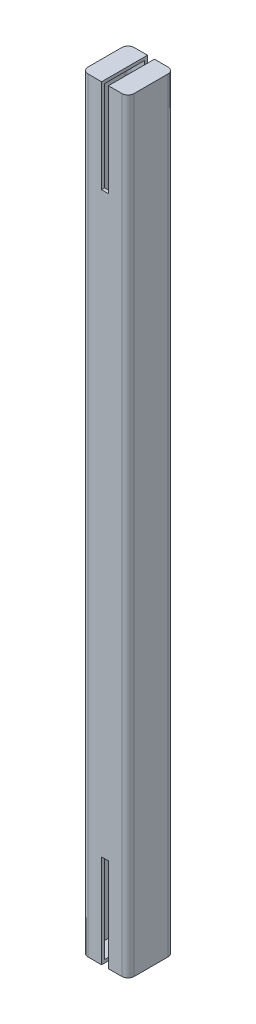
SolidWorks part; units mm, degrees
material "Q235B"
ref_plane "Front Plane" through (0, 0, 0) normal (0, 0, 1) x (1, 0, 0)
ref_plane "Top Plane" through (0, 0, 0) normal (0, 1, 0) x (1, 0, 0)
ref_plane "Right Plane" through (0, 0, 0) normal (1, 0, 0) x (0, 0, -1)
other "Configuration Table"
sketch "Sketch1" plane through (0, 0, 0) normal (0, 1, 0) x (1, 0, 0)
  line L0 (-22, 26) -> (22, 26)
  line L1 (-22, -30) -> (22, -30)
  line L2 (-30, -22) -> (-30, 22)
  line L3 (-22, 30) -> (22, 30)
  line L4 (30, -22) -> (30, 22)
  line L5 (-30, -30) -> (30, 30) construction
  line L6 (-30, 30) -> (30, -30) construction
  line L7 (26, -22) -> (26, 22)
  line L8 (-22, -26) -> (22, -26)
  line L9 (-26, -22) -> (-26, 22)
  arc A0 (-22, -30) -> (-30, -22) centre (-22, -22) cw
  arc A1 (22, -30) -> (30, -22) centre (22, -22) ccw
  arc A2 (22, 30) -> (30, 22) centre (22, 22) cw
  arc A3 (-30, 22) -> (-22, 30) centre (-22, 22) cw
  arc A4 (22, 26) -> (26, 22) centre (22, 22) cw
  arc A5 (22, -26) -> (26, -22) centre (22, -22) ccw
  arc A6 (-22, -26) -> (-26, -22) centre (-22, -22) cw
  arc A7 (-26, 22) -> (-22, 26) centre (-22, 22) cw
  point P0 (0, 0)
  dimension "D3" = 8
  dimension "D1" = 60
  dimension "D2" = 60
  dimension "D4" = 4
extrude "Boss-Extrude1" add sketch "Sketch1" along normal blind 998
sketch "Sketch2" plane through (0, 0, 30) normal (0, 0, 1) x (1, 0, 0)
  line L0 (-22, 998) -> (22, 998) construction
  line L1 (-4.5, 1120) -> (4.5, 1120)
  line L2 (-4.5, 1120) -> (-4.5, 876)
  line L3 (-4.5, 876) -> (4.5, 876)
  line L4 (4.5, 1120) -> (4.5, 876)
  line L5 (-4.5, 1120) -> (4.5, 876) construction
  line L6 (-4.5, 876) -> (4.5, 1120) construction
  line L7 (30, 998) -> (22, 998) construction
  line L9 (-4.5, -122) -> (4.5, -122)
  line L10 (-4.5, -122) -> (-4.5, 122)
  line L11 (-4.5, 122) -> (4.5, 122)
  line L12 (4.5, -122) -> (4.5, 122)
  line L13 (-4.5, -122) -> (4.5, 122) construction
  line L14 (-4.5, 122) -> (4.5, -122) construction
  point P0 (0, 998)
  point P9 (0, 0)
  dimension "D1" = 122
  dimension "D2" = 9
  dimension "D3" = 9
  dimension "D4" = 122
extrude "Cut-Extrude1" cut sketch "Sketch2" against normal through all both and the other way through all
sketch "Sketch3" plane through (0, 998, 0) normal (0, 1, 0) x (1, 0, 0)
  line L0 (-26, 22) -> (-26, -22) construction
  line L1 (-4.5, 26) -> (-26, 26)
  line L2 (-4.5, 26) -> (-4.5, -26)
  line L3 (-4.5, -26) -> (-26, -26)
  line L4 (-26, 26) -> (-26, -26)
  line L5 (-22, -26) -> (-4.5, -26) construction
  line L6 (0, 0) -> (0, 6.1347) construction
  line L7 (26, 26) -> (26, -26)
  line L8 (4.5, -26) -> (26, -26)
  line L9 (4.5, 26) -> (4.5, -26)
  line L10 (4.5, 26) -> (26, 26)
extrude "Boss-Extrude2" add sketch "Sketch3" against normal blind 4
sketch "Sketch4" plane through (0, 0, 0) normal (0, -1, 0) x (1, 0, 0)
  line L0 (-26, -22) -> (-26, 22) construction
  line L1 (-4.5, 26) -> (-26, 26)
  line L2 (-4.5, 26) -> (-4.5, -26)
  line L3 (-4.5, -26) -> (-26, -26)
  line L4 (-26, 26) -> (-26, -26)
  line L5 (-4.5, -26) -> (-22, -26) construction
  line L6 (0, 0) -> (0, 4.9739) construction
  line L7 (26, 26) -> (26, -26)
  line L8 (4.5, -26) -> (26, -26)
  line L9 (4.5, 26) -> (4.5, -26)
  line L10 (4.5, 26) -> (26, 26)
  dimension "D1" = 0
  dimension "D2" = 0
extrude "Boss-Extrude3" add sketch "Sketch4" against normal blind 4
